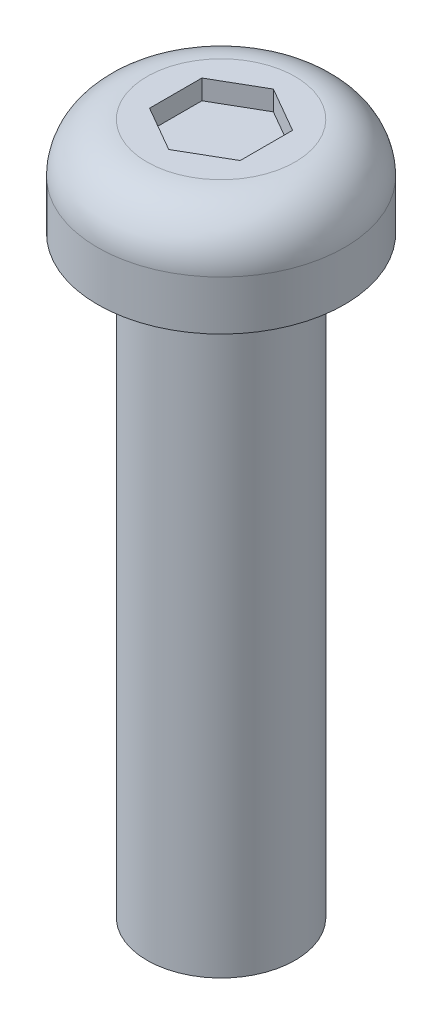
SolidWorks part; units mm, degrees
ref_plane "Front Plane" through (0, 0, 0) normal (0, 0, 1) x (1, 0, 0)
ref_plane "Top Plane" through (0, 0, 0) normal (0, 1, 0) x (1, 0, 0)
ref_plane "Right Plane" through (0, 0, 0) normal (1, 0, 0) x (0, 0, -1)
sketch "Sketch1" plane through (0, 0, 0) normal (0, 1, 0) x (1, 0, 0)
  circle A0 centre (0, 0) radius 0.75
  dimension "D1" = 1.5
extrude "Boss-Extrude1" add sketch "Sketch1" along normal blind 6
sketch "Sketch2" plane through (0, 6, 0) normal (0, 1, 0) x (1, 0, 0)
  circle A0 centre (0, 0) radius 1.25
  circle A1 centre (0, 0) radius 0.75 construction
  dimension "D1" = 0.5
extrude "Boss-Extrude2" add sketch "Sketch2" along normal blind 1
fillet "Fillet1" radius 0.5 1 edges at (0, 7, 1.25)
sketch "Sketch3" plane through (0, 7, 0) normal (0, 1, 0) x (1, 0, 0)
  line L1 (0, 0.5299) -> (-0.4589, 0.2649)
  line L2 (-0.4589, 0.2649) -> (-0.4589, -0.2649)
  line L3 (-0.4589, -0.2649) -> (0, -0.5299)
  line L4 (0, -0.5299) -> (0.4589, -0.2649)
  line L5 (0.4589, -0.2649) -> (0.4589, 0.2649)
  line L6 (0.4589, 0.2649) -> (0, 0.5299)
  circle A0 centre (0, 0) radius 0.4589 construction
extrude "Cut-Extrude1" cut sketch "Sketch3" against normal blind 0.2
